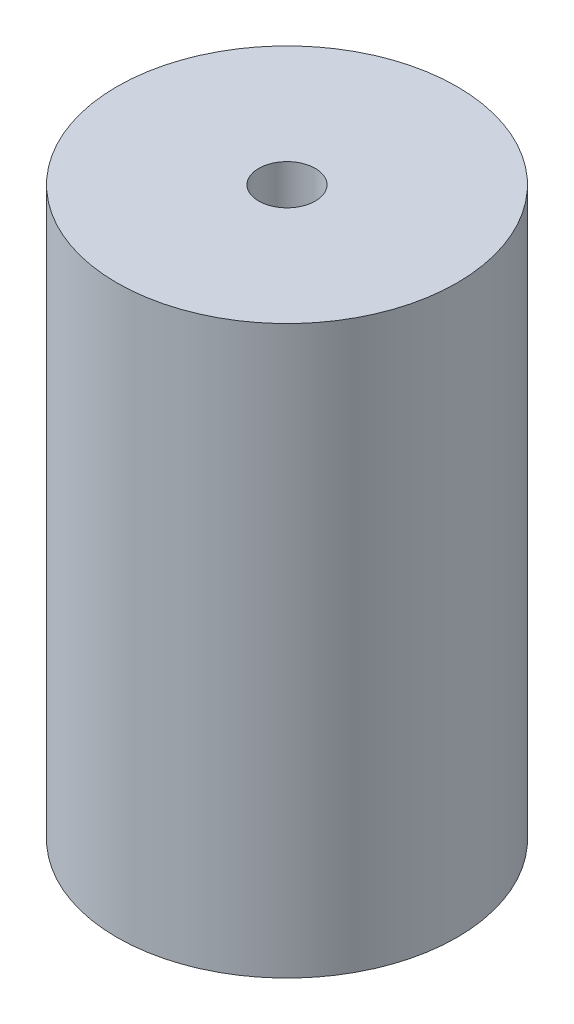
from build123d import *

# Parameters (mm, degrees)
SKETCH1_R           = 60
BOSS_EXTRUDE2_DEPTH = 200
SKETCH3_R           = 10
CUT_EXTRUDE2_DEPTH  = 40


with BuildPart() as part:
    # Sketch1 → Boss-Extrude2 (new body)
    with BuildSketch(Plane(origin=(0, 0, 0), x_dir=(1, 0, 0), z_dir=(0, 1, 0))):
        with Locations(Location((0, 0, 0), (0, 0, 270))):
            Circle(SKETCH1_R)
    extrude(amount=BOSS_EXTRUDE2_DEPTH)

    # Sketch3 → Cut-Extrude2 (cut)
    with BuildSketch(Plane(origin=(0, 200, 0), x_dir=(1, 0, 0), z_dir=(0, 1, 0))):
        with Locations(Location((0, 0, 0), (0, 0, 270))):
            Circle(SKETCH3_R)
    extrude(amount=-CUT_EXTRUDE2_DEPTH, mode=Mode.SUBTRACT)


solid = part.part
